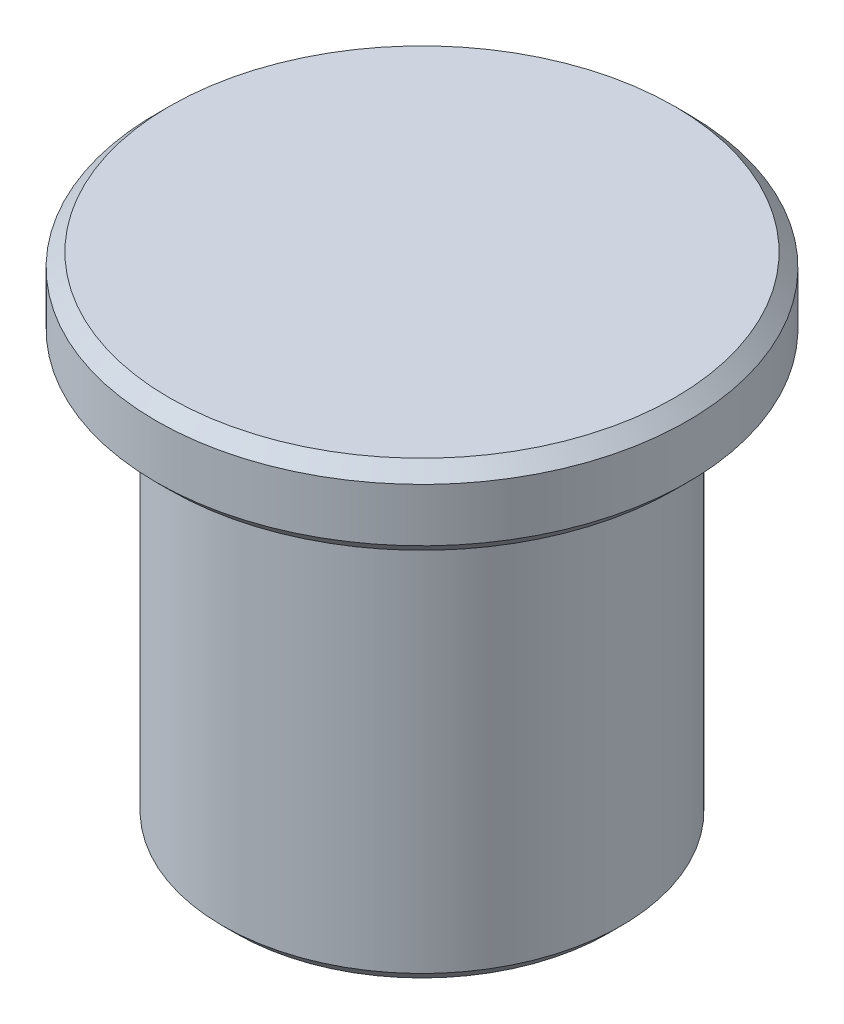
from build123d import *

# Parameters (mm, degrees)
CHAMFER1_SIZE = 0.5


with BuildPart() as part:
    # Sketch1 → Revolve1 (revolve)
    with BuildSketch(Plane.XY, mode=Mode.PRIVATE) as revolve1_sk:
        Polygon((1009, 204.198665167), (1009, 219.898665167), (1006.5, 219.898665167), (1006.5, 222.898665167), (1016.5, 222.898665167), (1016.5, 204.198665167), align=None)
    revolve(revolve1_sk.sketch.rotate(Axis((1016.5, 222.898665167, 0), (0, -1, 0)), 270), axis=Axis((1016.5, 222.898665167, 0), (0, -1, 0)))

    # Chamfer1
    chamfer1_edges = [part.edges().sort_by_distance(p)[0] for p in [
        (1016.5, 222.898665167, -10),
        (1016.5, 219.898665167, -10),
        (1016.5, 204.198665167, -7.5),
    ]]
    chamfer(chamfer1_edges, length=CHAMFER1_SIZE)


solid = part.part
